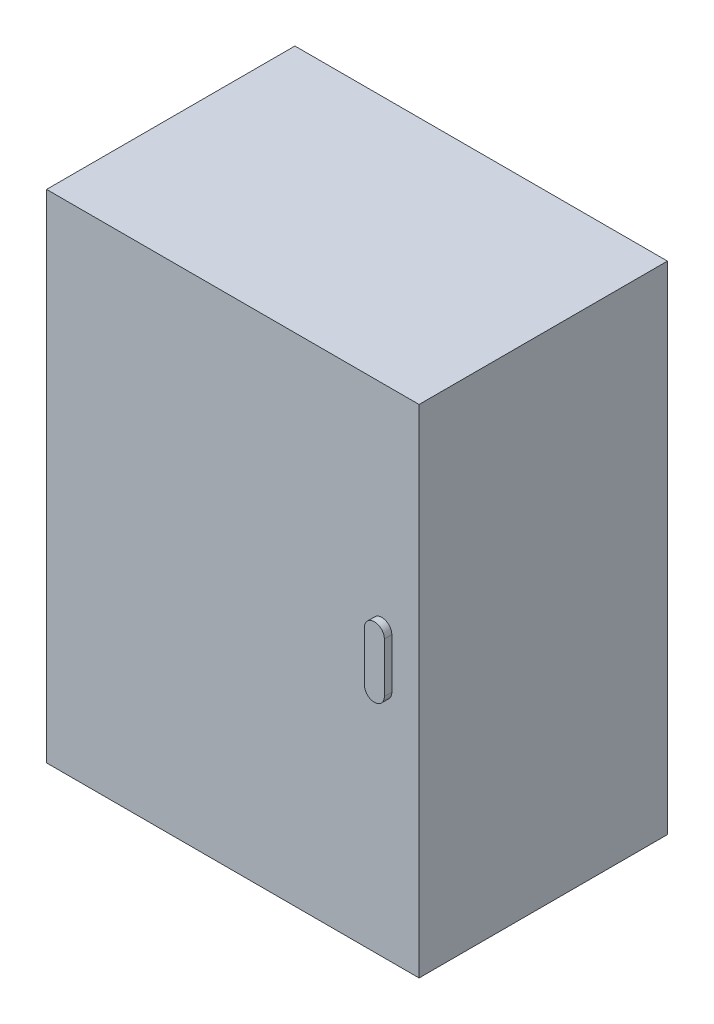
from build123d import *

# Parameters (mm, degrees)
SKETCH_1_W      = 300
SKETCH_1_H      = 400
EXTRUDE_1_DEPTH = 100
EXTRUDE_2_DEPTH = 6


with BuildPart() as part:
    # 草图1 → 凸台-拉伸1 (new, symmetric)
    with BuildSketch(Plane.XY):
        Rectangle(SKETCH_1_W, SKETCH_1_H)
    extrude(amount=EXTRUDE_1_DEPTH, both=True)

    # 草图2 → 凸台-拉伸2 (add)
    with BuildSketch(Plane.XY.offset(100)):
        with BuildLine():
            Line((128.030025312, 28.454220127), (128.030025312, -11.695906433))
            ThreePointArc((128.030025312, -11.695906433), (120, -19.725931745), (111.969974688, -11.695906433))
            Line((111.969974688, -11.695906433), (111.969974688, 28.454220127))
            ThreePointArc((111.969974688, 28.454220127), (120, 36.484245439), (128.030025312, 28.454220127))
        make_face()
    extrude(amount=EXTRUDE_2_DEPTH)


solid = part.part
